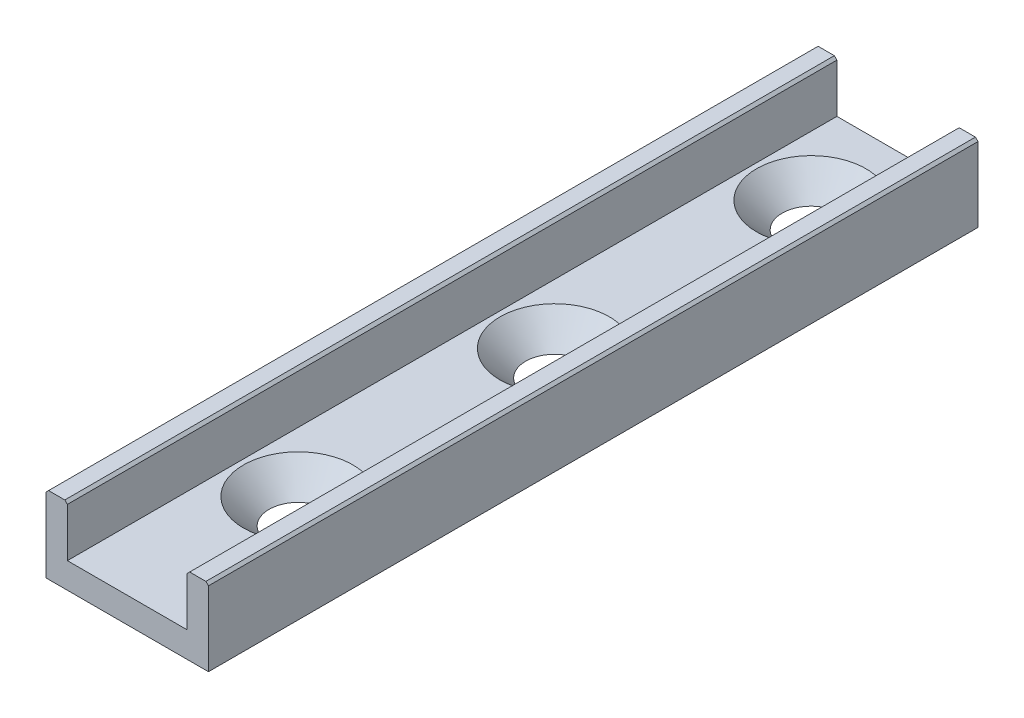
SolidWorks part; units mm, degrees
ref_plane "Front Plane" through (0, 0, 0) normal (0, 0, 1) x (1, 0, 0)
ref_plane "Top Plane" through (0, 0, 0) normal (0, 1, 0) x (1, 0, 0)
ref_plane "Right Plane" through (0, 0, 0) normal (1, 0, 0) x (0, 0, -1)
sketch "Sketch1" plane through (0, 0, 0) normal (0, 0, 1) x (1, 0, 0)
  line L0 (-7, 4.5) -> (-7, -1.5)
  line L1 (-9.5, -4.5) -> (9.5, -4.5)
  line L2 (-9.5, -4.5) -> (-9.5, 4.5)
  line L3 (-9.5, 4.5) -> (-7, 4.5)
  line L4 (9.5, -4.5) -> (9.5, 4.5)
  line L5 (-9.5, -4.5) -> (9.5, 4.5) construction
  line L6 (-9.5, 4.5) -> (9.5, -4.5) construction
  line L7 (-7, -1.5) -> (7, -1.5)
  line L8 (7, -1.5) -> (7, 4.5)
  line L9 (7, 4.5) -> (9.5, 4.5)
  point P0 (0, 0)
  dimension "D1" = 2.5
  dimension "D2" = 2.5
  dimension "D3" = 3
  dimension "D4" = 9
  dimension "D5" = 14
extrude "Boss-Extrude1" add sketch "Sketch1" along normal blind 90
hole_wizard "Hole size per hex socket lobed semi-countersunk screw type1" positions "Sketch4" profile "Sketch5" countersink size "M6" standard "GB" end condition through all
sketch "Sketch4" plane through (0, -1.5, 0) normal (0, 1, 0) x (1, 0, 0)
  line L0 (7, 0) -> (-7, 0) construction
  point P0 (0, -10)
  point P6 (0, -40)
  dimension "D1" = 10
  dimension "D2" = 30
sketch "Sketch5" plane through (0, -1.5, 10) normal (1, 0, 0) x (0, 0, 1)
  line L0 (0, 0) -> (0, 3)
  line L1 (0, 3) -> (3.3, 3)
  line L2 (3.3, 3) -> (3.3, 3.1)
  line L3 (3.3, 3.1) -> (6.4, 0)
  line L5 (6.4, 0) -> (0, 0)
  line L6 (-3.3, 3.1) -> (-6.4, 0) construction
  line L11 (0, -6.35) -> (0, 107.95) construction
  dimension "通孔孔直径" = 6.6
  dimension "通孔孔深度" = 3
  dimension "近端锥形沉头孔直径" = 12.8
  dimension "近端锥形沉头孔角度" = 90
pattern_linear "LPattern1" count 2 spacing 30 along (0, 0, 1) of "Hole size per hex socket lobed semi-countersunk screw type1"
chamfer "Chamfer1" distance 0.3 angle 45 4 edges at (-9.5, 4.5, 45) (9.5, 4.5, 45) (-7, 4.5, 45) (7, 4.5, 45)
